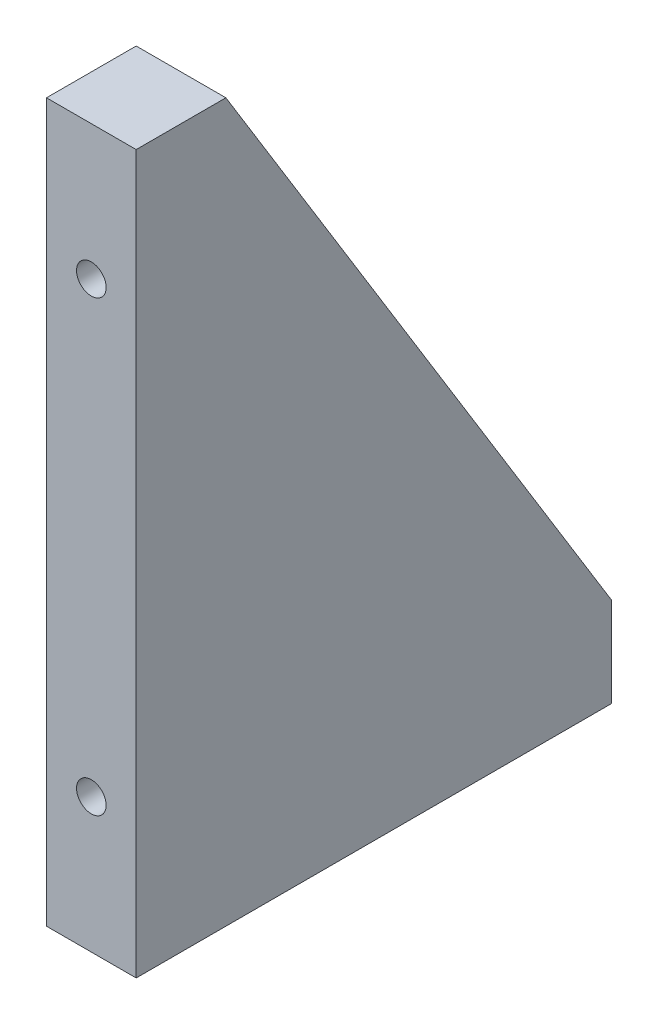
SolidWorks part; units mm, degrees
material "AL6061"
ref_plane "Front Plane" through (0, 0, 0) normal (0, 0, 1) x (1, 0, 0)
ref_plane "Top Plane" through (0, 0, 0) normal (0, 1, 0) x (1, 0, 0)
ref_plane "Right Plane" through (0, 0, 0) normal (1, 0, 0) x (0, 0, -1)
sketch "Sketch1" plane through (0, 0, 0) normal (1, 0, 0) x (0, 0, -1)
  line L0 (0, 0) -> (0, 80)
  line L1 (0, 80) -> (10, 80)
  line L2 (10, 80) -> (53, 10)
  line L3 (53, 10) -> (53, 0)
  line L4 (53, 0) -> (0, 0)
  dimension "D1" = 53
  dimension "D2" = 10
  dimension "D3" = 10
  dimension "D4" = 80
extrude "Boss-Extrude1" add sketch "Sketch1" along normal blind 10
hole_wizard "M4 Tapped Hole1" positions "Sketch4" profile "Sketch5" tap size "M4" standard "GB"
sketch "Sketch4" plane through (0, 0, 0) normal (0, 0, 1) x (1, 0, 0)
  line L0 (5, 80) -> (5, 0) construction
  line L1 (10, 80) -> (0, 80) construction
  line L2 (10, 0) -> (0, 0) construction
  line L3 (0, 40) -> (10, 40) construction
  line L4 (0, 80) -> (0, 0) construction
  line L5 (10, 80) -> (10, 0) construction
  point P0 (5, 65)
  point P11 (5, 15)
  dimension "D1" = 50
sketch "Sketch5" plane through (5, 65, 0) normal (1, 0, 0) x (0, -1, 0)
  line L0 (0, 0) -> (0, 11.0914)
  line L1 (0, 11.0914) -> (1.65, 10.1)
  line L2 (1.65, 10.1) -> (1.65, 0)
  line L5 (1.65, 0) -> (0, 0)
  line L10 (0, 11.0914) -> (-1.65, 10.1) construction
  line L11 (0, -6.35) -> (0, 107.95) construction
  dimension "螺纹孔钻头直径" = 3.3
  dimension "螺纹孔钻头深度" = 10.1
  dimension "导头角度" = 118
cosmetic thread "Cosmetic thread1" parameters "D1"=8, "D2"=4
cosmetic thread "Cosmetic thread2" parameters "D1"=8, "D2"=4
hole_wizard "M4 Tapped Hole2" positions "Sketch6" profile "Sketch7" tap size "M4" standard "GB"
sketch "Sketch6" plane through (0, 0, 0) normal (0, -1, 0) x (-1, 0, 0)
  point P0 (-5, 43)
  point P3 (-5, 8)
sketch "Sketch7" plane through (5, 0, -43) normal (1, 0, 0) x (0, 0, -1)
  line L0 (0, 0) -> (0, 11.0914)
  line L1 (0, 11.0914) -> (1.65, 10.1)
  line L2 (1.65, 10.1) -> (1.65, 0)
  line L5 (1.65, 0) -> (0, 0)
  line L10 (0, 11.0914) -> (-1.65, 10.1) construction
  line L11 (0, -6.35) -> (0, 107.95) construction
  dimension "螺纹孔钻头直径" = 3.3
  dimension "螺纹孔钻头深度" = 10.1
  dimension "导头角度" = 118
cosmetic thread "Cosmetic thread3" parameters "D1"=8, "D2"=4
cosmetic thread "Cosmetic thread4" parameters "D1"=8, "D2"=4
